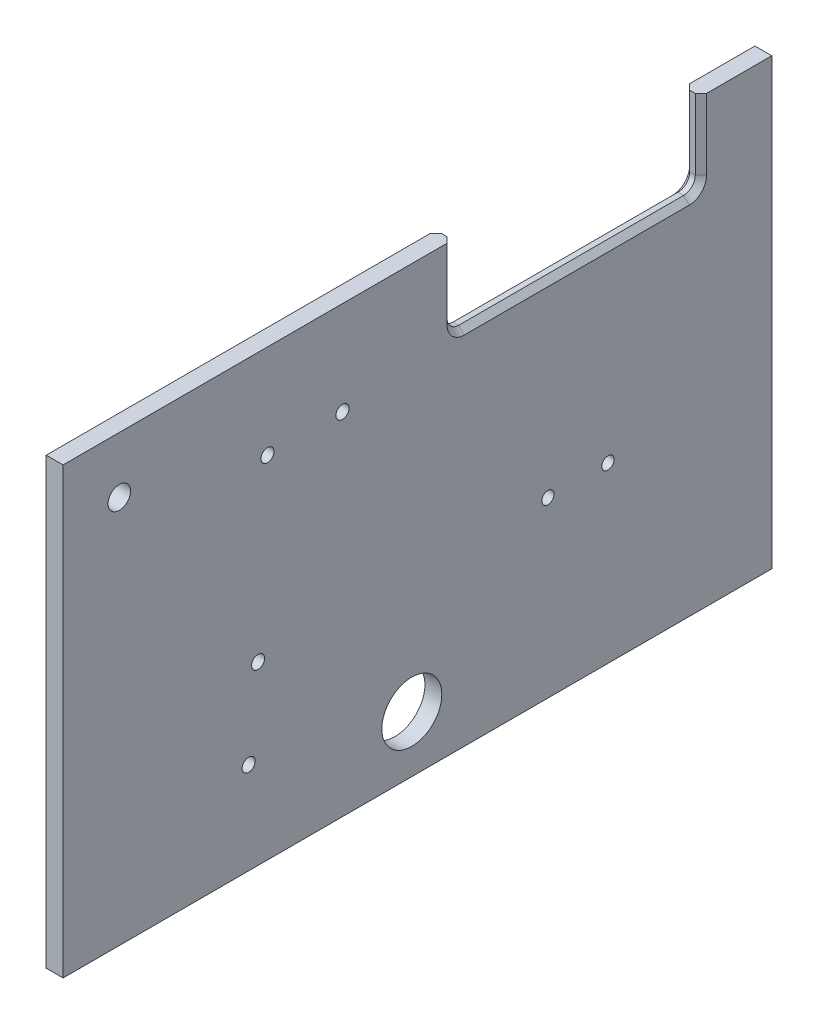
from build123d import *

# Parameters (mm, degrees)
BOSS_EXTRUDE1_DEPTH = 22.5
SKETCH2_R           = 30
SKETCH2_R_2         = 17.5
SKETCH2_R_3         = 80
CUT_EXTRUDE1_DEPTH  = 1812.9464672
FILLET1_R           = 31
CHAMFER1_SIZE       = 15
SKETCH3_R           = 16.5
CUT_EXTRUDE2_DEPTH  = 159


with BuildPart() as part:
    # Sketch1 → Boss-Extrude1 (new, symmetric)
    with BuildSketch(Plane(origin=(0, 0, 0), x_dir=(0, 0, -1), z_dir=(1, 0, 0))):
        Polygon((0, 0), (520, 0), (520, 1185), (331, 1185), (331, 965), (-331, 965), (-331, 1185), (-1370, 1185), (-1370, 0), align=None)
    extrude(amount=BOSS_EXTRUDE1_DEPTH, both=True)

    # Sketch2 → Cut-Extrude1 (cut, through all)
    with BuildSketch(Plane(origin=(22.5, 0, 0), x_dir=(0, 0, -1), z_dir=(1, 0, 0))):
        with Locations((-1220, 1035)):
            Circle(SKETCH2_R)
        with Locations((-825, 935)):
            Circle(SKETCH2_R_2)
        with Locations((-625, 935)):
            Circle(SKETCH2_R_2)
        with Locations((-850, 470)):
            Circle(SKETCH2_R_2)
        with Locations((-875, 245)):
            Circle(SKETCH2_R_2)
        with Locations((-440, 150)):
            Circle(SKETCH2_R_3)
    extrude(amount=-CUT_EXTRUDE1_DEPTH, mode=Mode.SUBTRACT)

    # Fillet1
    fillet1_edges = [part.edges().sort_by_distance(p)[0] for p in [
        (0, 965, 331),
        (0, 965, -331),
    ]]
    fillet(fillet1_edges, radius=FILLET1_R)

    # Chamfer1
    chamfer1_edges = [part.edges().sort_by_distance(p)[0] for p in [
        (-22.5, 1090.5, -331),
        (22.5, 1090.5, -331),
        (-22.5, 965, 0),
        (22.5, 965, 0),
        (-22.5, 1090.5, 331),
        (22.5, 1090.5, 331),
        (-22.5, 974.079689783, -321.920310217),
        (22.5, 974.079689783, -321.920310217),
        (-22.5, 974.079689783, 321.920310217),
        (22.5, 974.079689783, 321.920310217),
    ]]
    chamfer(chamfer1_edges, length=CHAMFER1_SIZE)

    # Sketch3 → Cut-Extrude2 (cut)
    with BuildSketch(Plane(origin=(22.5, 0, 0), x_dir=(0, 0, -1), z_dir=(1, 0, 0))):
        with Locations((-77, 463)):
            Circle(SKETCH3_R)
        with Locations((83, 463)):
            Circle(SKETCH3_R)
    extrude(amount=-CUT_EXTRUDE2_DEPTH, mode=Mode.SUBTRACT)


solid = part.part
